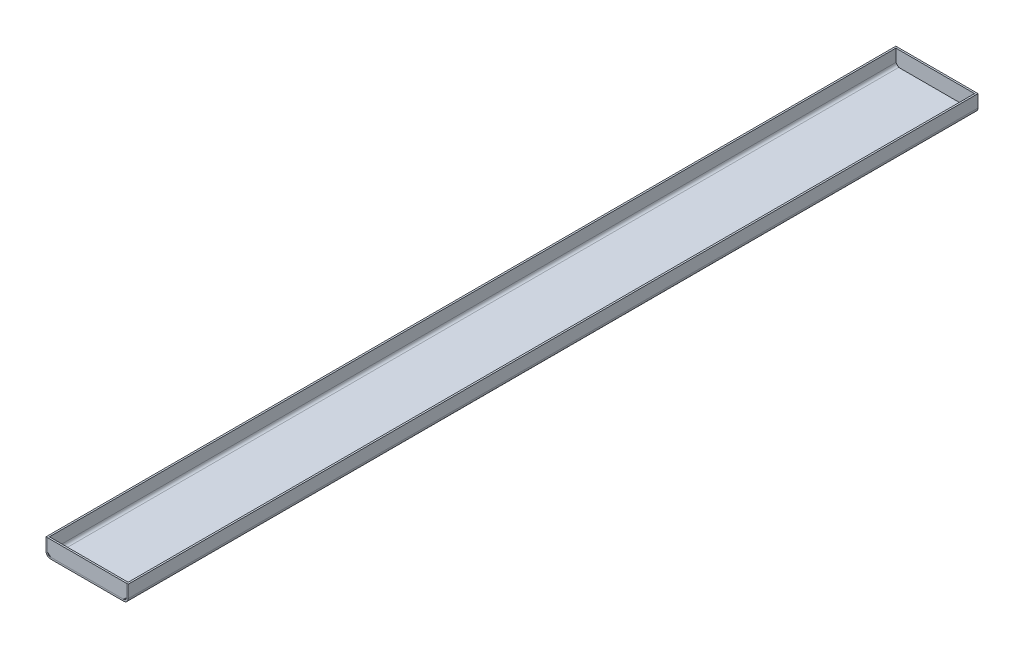
SolidWorks part; units mm, degrees
material "1023 碳钢板 (SS)"
ref_plane "Front Plane" through (0, 0, 0) normal (0, 0, 1) x (1, 0, 0)
ref_plane "Top Plane" through (0, 0, 0) normal (0, 1, 0) x (1, 0, 0)
ref_plane "Right Plane" through (0, 0, 0) normal (1, 0, 0) x (0, 0, -1)
sketch "Sketch1" plane through (0, 0, 0) normal (0, 0, 1) x (1, 0, 0)
  line L0 (0, 0) -> (0, -22)
  line L1 (8, -30) -> (137, -30)
  line L2 (145, -22) -> (145, 0)
  line L3 (3, 0) -> (3, -22)
  line L4 (8, -27) -> (137, -27)
  line L5 (142, -22) -> (142, 0)
  line L6 (0, 0) -> (3, 0)
  line L7 (145, 0) -> (142, 0)
  arc A0 (137, -30) -> (145, -22) centre (137, -22) ccw
  arc A1 (0, -22) -> (8, -30) centre (8, -22) ccw
  arc A2 (3, -22) -> (8, -27) centre (8, -22) ccw
  arc A3 (137, -27) -> (142, -22) centre (137, -22) ccw
  point P7 (145, -30)
  point P10 (0, -30)
  dimension "D3" = 8
  dimension "D1" = 30
  dimension "D2" = 145
  dimension "D4" = 3
extrude "Boss-Extrude1" add sketch "Sketch1" along normal blind 1500 contours L7 L5 A3 L4 A2 L3 L6 L0 A1 L1 A0 L2
sketch "Sketch3" plane through (0, 0, 1500) normal (0, 0, 1) x (1, 0, 0)
  line L0 (3, 0) -> (142, 0)
  line L1 (142, 0) -> (142, -22)
  line L2 (137, -27) -> (8, -27)
  line L3 (3, -22) -> (3, 0)
  line L4 (8, -27) -> (3, -22)
  line L5 (142, -22) -> (137, -27)
  point P5 (142, -27)
  point P6 (3, -27)
extrude "Boss-Extrude2" add sketch "Sketch3" against normal blind 3 separate body contours L3 L0 L1 L5 L2 L4
sketch "Sketch4" plane through (0, 0, 0) normal (0, 0, -1) x (-1, 0, 0)
  line L0 (-142, 0) -> (-3, 0)
  line L1 (-3, 0) -> (-3, -22)
  line L2 (-8, -27) -> (-137, -27)
  line L3 (-142, -22) -> (-142, 0)
  line L4 (-137, -27) -> (-142, -22)
  line L5 (-3, -22) -> (-8, -27)
  point P5 (-3, -27)
  point P6 (-142, -27)
extrude "Boss-Extrude3" add sketch "Sketch4" against normal blind 3 separate body
